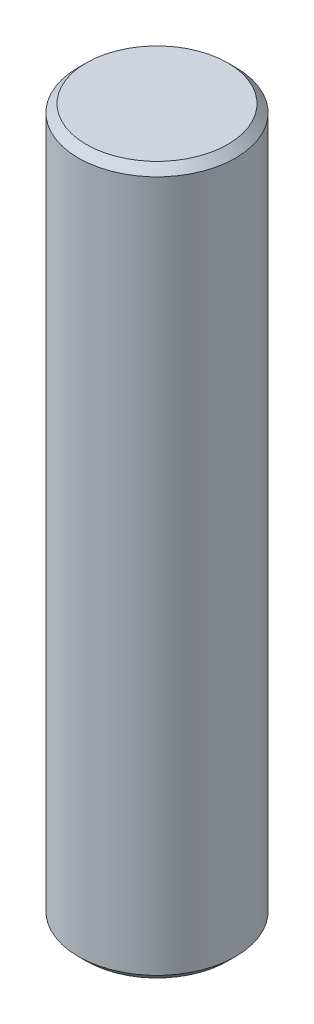
SolidWorks part; units mm, degrees
material "SUS304"
ref_plane "Front Plane" through (0, 0, 0) normal (0, 0, 1) x (1, 0, 0)
ref_plane "Top Plane" through (0, 0, 0) normal (0, 1, 0) x (1, 0, 0)
ref_plane "Right Plane" through (0, 0, 0) normal (1, 0, 0) x (0, 0, -1)
sketch "Sketch1" plane through (0, 0, 0) normal (0, 1, 0) x (1, 0, 0)
  circle A0 centre (0, 0) radius 5
  dimension "D1" = 10
extrude "Boss-Extrude1" add sketch "Sketch1" along normal blind 45
hole_wizard "M5 Tapped Hole1" positions "3DSketch1" profile "Sketch2" tap size "M5" standard "GB"
sketch3d "3DSketch1"
  point P0 (0, 0, 0)
  dimension "D1" = 0
sketch "Sketch2" plane through (0, 0, 0) normal (1, 0, 0) x (0, 0, -1)
  line L0 (0, 0) -> (0, 13.6618)
  line L1 (0, 13.6618) -> (2.1, 12.4)
  line L2 (2.1, 12.4) -> (2.1, 0)
  line L5 (2.1, 0) -> (0, 0)
  line L10 (0, 13.6618) -> (-2.1, 12.4) construction
  line L11 (0, -6.35) -> (0, 107.95) construction
  dimension "螺纹孔钻头直径" = 4.2
  dimension "螺纹孔钻头深度" = 12.4
  dimension "导头角度" = 118
cosmetic thread "Cosmetic Thread1" parameters "D1"=10, "D2"=5
chamfer "Chamfer1" distance 0.5 angle 45 2 edges at (0, 45, 5) (0, 0, 5)
